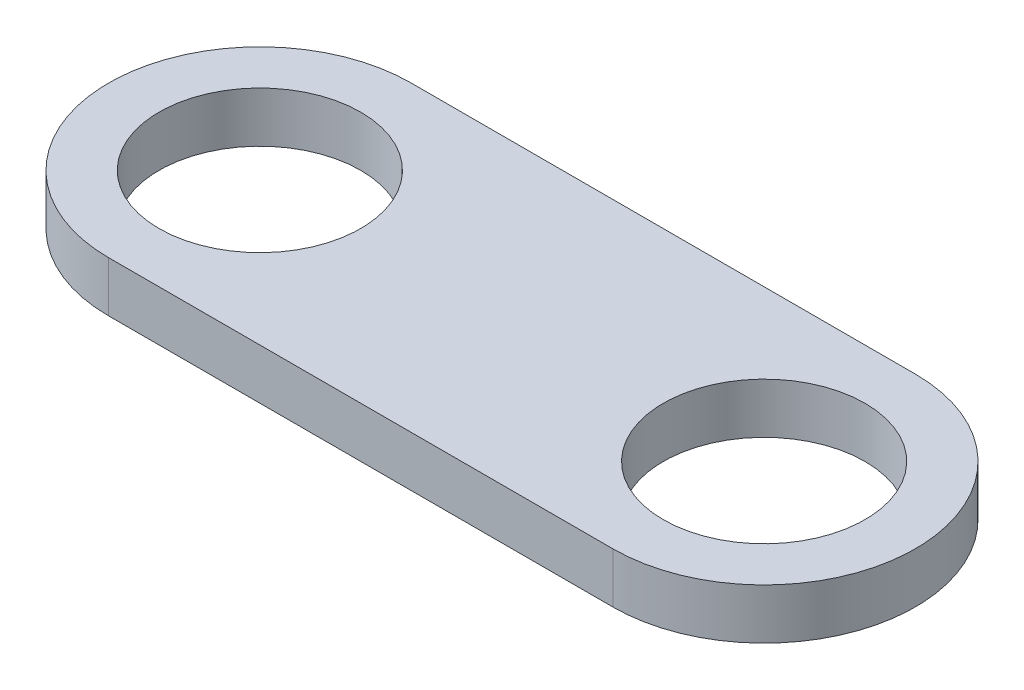
from build123d import *

# Parameters (mm, degrees)
SKETCH_1_R      = 20
EXTRUDE_1_DEPTH = 10


with BuildPart() as part:
    # 草图1 → 凸台-拉伸1 (new body)
    with BuildSketch(Plane(origin=(0, 0, 0), x_dir=(1, 0, 0), z_dir=(0, 1, 0))):
        with BuildLine():
            Line((-50, 30), (50, 30))
            ThreePointArc((50, 30), (80, 0), (50, -30))
            Line((50, -30), (-50, -30))
            ThreePointArc((-50, -30), (-80, 0), (-50, 30))
        make_face()
        with Locations(Location((50, 0, 0), (0, 0, 270))):
            Circle(SKETCH_1_R, mode=Mode.SUBTRACT)
        with Locations(Location((-50, 0, 0), (0, 0, 270))):
            Circle(SKETCH_1_R, mode=Mode.SUBTRACT)
    extrude(amount=EXTRUDE_1_DEPTH)


solid = part.part
